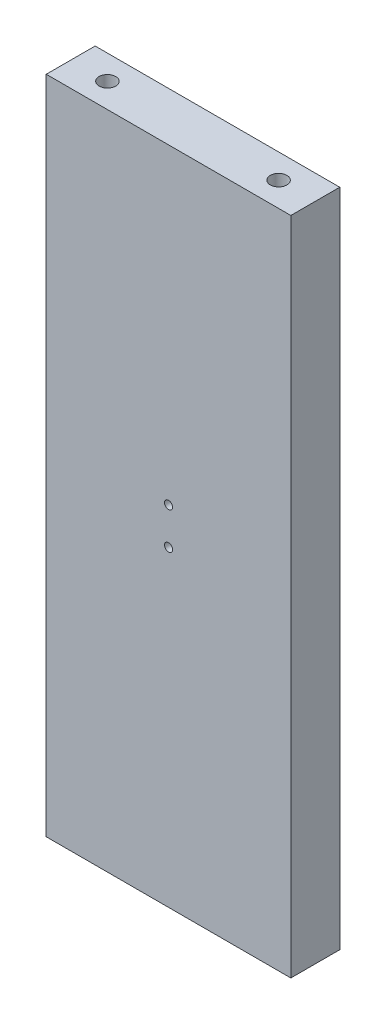
from build123d import *

# Parameters (mm, degrees)
SKETCH1_W                       = 100
SKETCH1_H                       = 270
BOSS_EXTRUDE1_DEPTH             = 20
M8_TAPPED_HOLE1_D               = 6.8
M8_TAPPED_HOLE1_DEPTH           = 19.75
M8_TAPPED_HOLE1_TIP             = 2.042926105
M8_TAPPED_HOLE1_ON_FACE_2_D     = 6.8
M8_TAPPED_HOLE1_ON_FACE_2_DEPTH = 19.75
M8_TAPPED_HOLE1_ON_FACE_2_TIP   = 2.042926105
M4_TAPPED_HOLE2_D               = 3.3
M4_TAPPED_HOLE2_DEPTH           = 10.1
M4_TAPPED_HOLE2_TIP             = 0.991420021
M4_TAPPED_HOLE1_D               = 3.3
M4_TAPPED_HOLE1_DEPTH           = 10.1
M4_TAPPED_HOLE1_TIP             = 0.991420021


with BuildPart() as part:
    # Sketch1 → Boss-Extrude1 (new body)
    with BuildSketch(Plane.XY):
        with Locations((50, -135)):
            Rectangle(SKETCH1_W, SKETCH1_H)
    extrude(amount=BOSS_EXTRUDE1_DEPTH)

    # M8 Tapped Hole1
    with Locations(Plane(origin=(15, 0, 10), x_dir=(0, 0, 1), z_dir=(0, 1, 0))):
        with Locations((0, 0), (0, 70)):
            Hole(M8_TAPPED_HOLE1_D / 2, depth=M8_TAPPED_HOLE1_DEPTH)
            with Locations((0, 0, -(M8_TAPPED_HOLE1_DEPTH + M8_TAPPED_HOLE1_TIP / 2))):  # 118° drill point
                Cone(0, M8_TAPPED_HOLE1_D / 2, M8_TAPPED_HOLE1_TIP, mode=Mode.SUBTRACT)

    # M8 Tapped Hole1 on face 2
    with Locations(Plane(origin=(15, -270, 10), x_dir=(0, 0, -1), z_dir=(0, -1, 0))):
        with Locations((0, 0), (0, 70)):
            Hole(M8_TAPPED_HOLE1_ON_FACE_2_D / 2, depth=M8_TAPPED_HOLE1_ON_FACE_2_DEPTH)
            with Locations((0, 0, -(M8_TAPPED_HOLE1_ON_FACE_2_DEPTH + M8_TAPPED_HOLE1_ON_FACE_2_TIP / 2))):  # 118° drill point
                Cone(0, M8_TAPPED_HOLE1_ON_FACE_2_D / 2, M8_TAPPED_HOLE1_ON_FACE_2_TIP, mode=Mode.SUBTRACT)

    # M4 Tapped Hole2
    with Locations(Plane.XY.offset(20)):
        with Locations((50, -127.5), (50, -142.5)):
            Hole(M4_TAPPED_HOLE2_D / 2, depth=M4_TAPPED_HOLE2_DEPTH)
            with Locations((0, 0, -(M4_TAPPED_HOLE2_DEPTH + M4_TAPPED_HOLE2_TIP / 2))):  # 118° drill point
                Cone(0, M4_TAPPED_HOLE2_D / 2, M4_TAPPED_HOLE2_TIP, mode=Mode.SUBTRACT)

    # M4 Tapped Hole1
    with Locations(Plane(origin=(0, 0, 0), x_dir=(-1, 0, 0), z_dir=(0, 0, -1))):
        with Locations((-60, -55), (-60, -115), (-60, -175)):
            Hole(M4_TAPPED_HOLE1_D / 2, depth=M4_TAPPED_HOLE1_DEPTH)
            with Locations((0, 0, -(M4_TAPPED_HOLE1_DEPTH + M4_TAPPED_HOLE1_TIP / 2))):  # 118° drill point
                Cone(0, M4_TAPPED_HOLE1_D / 2, M4_TAPPED_HOLE1_TIP, mode=Mode.SUBTRACT)


solid = part.part
